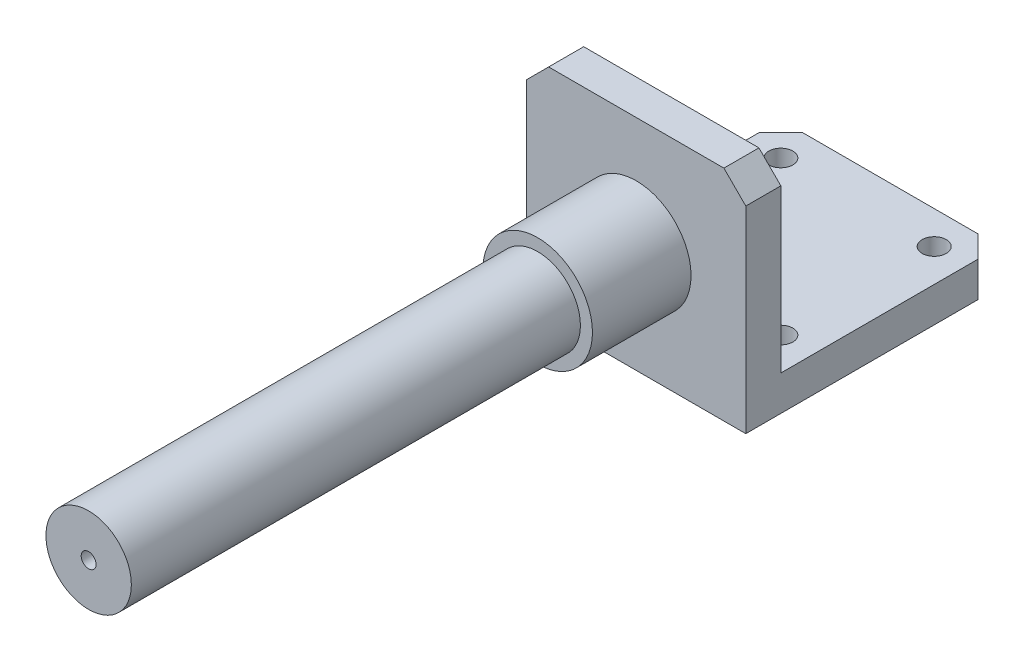
SolidWorks part; units mm, degrees
material "Q235-A"
ref_plane "前视基准面" through (0, 0, 0) normal (0, 0, 1) x (1, 0, 0)
ref_plane "上视基准面" through (0, 0, 0) normal (0, 1, 0) x (1, 0, 0)
ref_plane "右视基准面" through (0, 0, 0) normal (1, 0, 0) x (0, 0, -1)
sketch "草图1" plane through (0, 0, 0) normal (0, 0, 1) x (1, 0, 0)
  line L1 (-50, -50) -> (50, -50)
  line L2 (-50, -50) -> (-50, 50)
  line L3 (-50, 50) -> (50, 50)
  line L4 (50, -50) -> (50, 50)
  line L5 (-50, -50) -> (50, 50) construction
  line L6 (-50, 50) -> (50, -50) construction
  point P0 (0, 0)
  dimension "D1" = 100
  dimension "D2" = 100
extrude "凸台-拉伸1" add sketch "草图1" along normal blind 16
sketch "草图2" plane through (0, 0, 16) normal (0, 0, 1) x (1, 0, 0)
  circle A0 centre (0, 0) radius 25
  dimension "D1" = 50
extrude "凸台-拉伸2" add sketch "草图2" along normal blind 250
sketch "草图3" plane through (0, 0, 266) normal (0, 0, 1) x (1, 0, 0)
  circle A0 centre (0, 0) radius 19.5
  dimension "D1" = 39
extrude "切除-拉伸1" cut sketch "草图3" against normal blind 205 flip side to cut
sketch "草图8" plane through (0, 0, 0) normal (0, 0, -1) x (-1, 0, 0)
  line L0 (-50, -50) -> (-50, 50) construction
  line L1 (50, -50) -> (-50, -50)
  line L2 (50, -50) -> (50, -34)
  line L3 (50, -34) -> (-50, -34)
  line L4 (-50, -50) -> (-50, -34)
  dimension "D1" = 16
extrude "凸台-拉伸3" add sketch "草图8" along normal blind 100
hole_wizard "M8 螺纹孔1" positions "草图4" profile "草图5" tap size "M8" standard "GB"
sketch "草图4" plane through (0, 0, 266) normal (0, 0, 1) x (1, 0, 0)
  point P0 (0, 0)
cosmetic thread "孔螺蚊线1" parameters "D1"=16, "D2"=8
sketch "草图5" plane through (0, 0, 266) normal (1, 0, 0) x (0, -1, 0)
  line L0 (0, 0) -> (0, 21.7929)
  line L1 (0, 21.7929) -> (3.4, 19.75)
  line L2 (3.4, 19.75) -> (3.4, 0)
  line L5 (3.4, 0) -> (0, 0)
  line L10 (0, 21.7929) -> (-3.4, 19.75) construction
  line L11 (0, -6.35) -> (0, 107.95) construction
  dimension "螺纹孔钻头直径" = 6.8
  dimension "螺纹孔钻头深度" = 19.75
  dimension "导头角度" = 118
hole_wizard "M10 间隙孔1" positions "草图6" profile "草图7" hole size "M10" standard "GB" end condition through all
sketch "草图6" plane through (0, -34, -18) normal (0, 1, 0) x (1, 0, 0)
  line L7 (-50, 82) -> (-50, -18) construction
  line L8 (-50, 82) -> (50, 82) construction
  point P0 (-35, 67)
  point P2 (35, 67)
  point P4 (35, -3)
  point P6 (-35, -3)
  dimension "D1" = 70
  dimension "D2" = 70
  dimension "D3" = 15
  dimension "D4" = 15
sketch "草图7" plane through (-35, -34, -85) normal (1, 0, 0) x (0, 0, 1)
  line L0 (0, 0) -> (0, 16)
  line L1 (0, 16) -> (5.5, 16)
  line L2 (5.5, 16) -> (5.5, 0)
  line L5 (5.5, 0) -> (0, 0)
  line L11 (0, -6.35) -> (0, 107.95) construction
  dimension "通孔孔直径" = 11
  dimension "通孔孔深度" = 16
chamfer "倒角1" distance 10 angle 45 4 edges at (50, 50, 8) (-50, 50, 8) (-50, -42, -100) (50, -42, -100)
